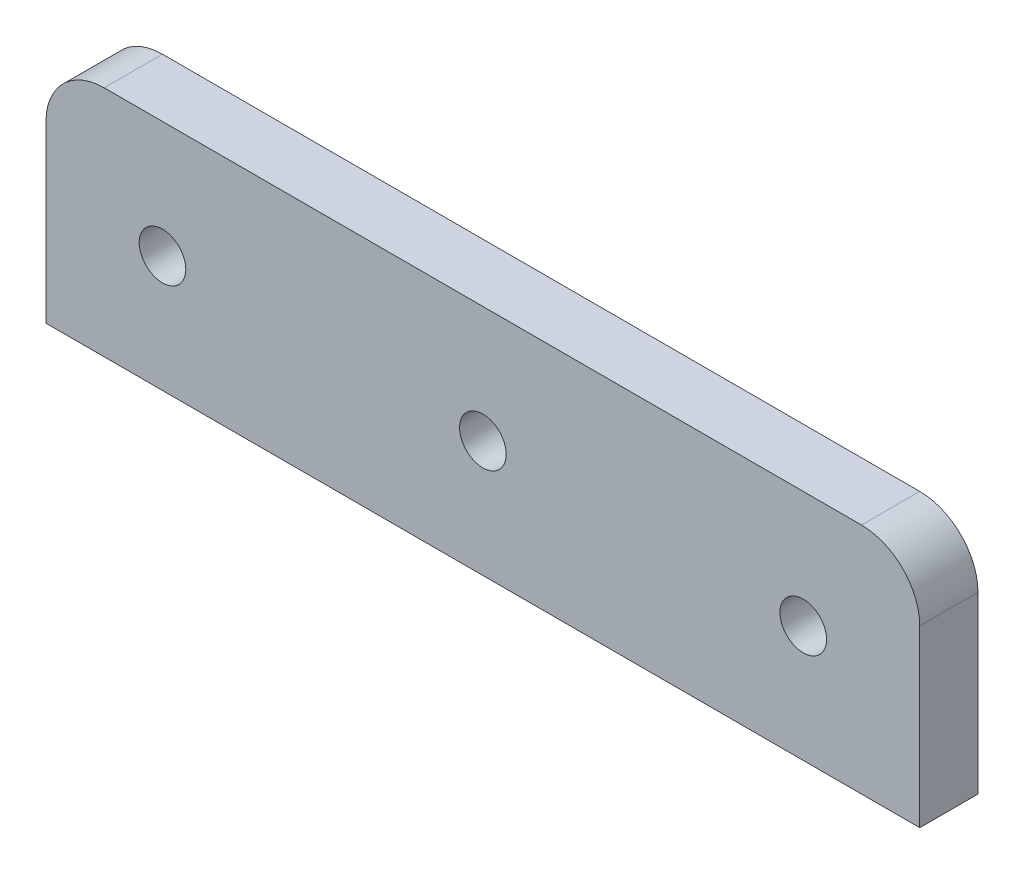
SolidWorks part; units mm, degrees
material "普通碳钢"
ref_plane "Front Plane" through (0, 0, 0) normal (0, 0, 1) x (1, 0, 0)
ref_plane "Top Plane" through (0, 0, 0) normal (0, 1, 0) x (1, 0, 0)
ref_plane "Right Plane" through (0, 0, 0) normal (1, 0, 0) x (0, 0, -1)
sketch "Sketch1" plane through (0, 0, 0) normal (0, 0, 1) x (1, 0, 0)
  line L0 (10, -10) -> (65, -10) construction
  line L1 (0, 0) -> (75, 0)
  line L2 (0, 0) -> (0, -20)
  line L3 (0, -20) -> (75, -20)
  line L4 (75, 0) -> (75, -20)
  line L5 (0, 0) -> (75, -20) construction
  line L6 (0, -20) -> (75, 0) construction
  circle A0 centre (10, -10) radius 2
  circle A2 centre (65, -10) radius 2
  circle A3 centre (37.5, -10) radius 2
  point P4 (37.5, -10)
  point P12 (37.5, -10)
  point P13 (37.5, -10)
  dimension "D3" = 4
  dimension "D1" = 20
  dimension "D2" = 75
  dimension "D4" = 55
  dimension "D6" = 10
extrude "Boss-Extrude1" add sketch "Sketch1" along normal blind 5
fillet "Fillet1" radius 5 2 edges at (75, 0, 2.5) (0, 0, 2.5)
